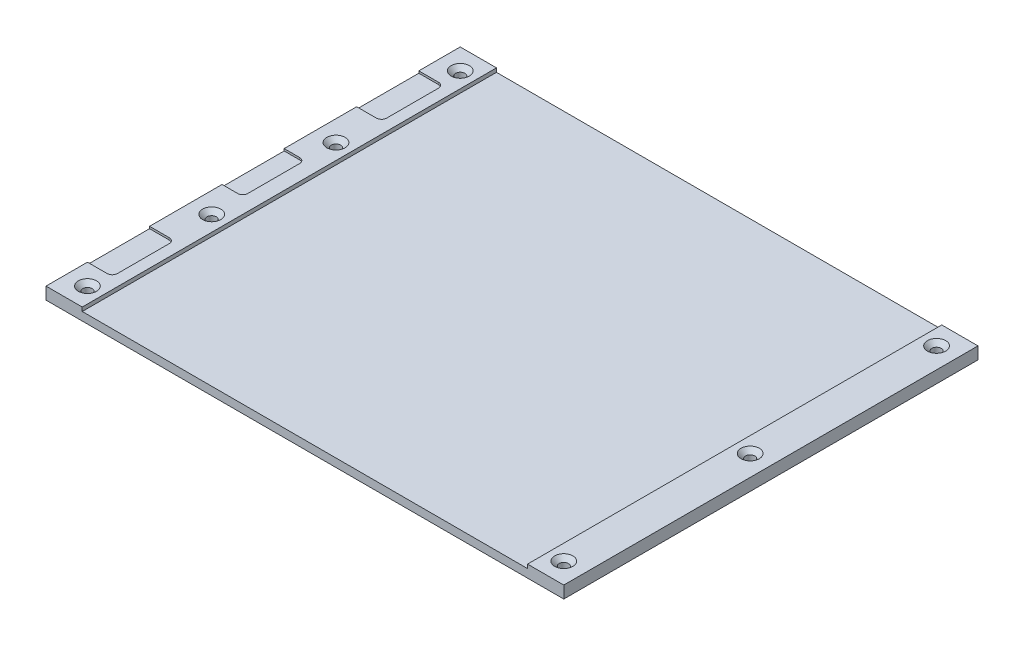
SolidWorks part; units mm, degrees
material "玻璃"
ref_plane "Front" through (0, 0, 0) normal (0, 0, 1) x (1, 0, 0)
ref_plane "Top" through (0, 0, 0) normal (0, 1, 0) x (1, 0, 0)
ref_plane "Right" through (0, 0, 0) normal (1, 0, 0) x (0, 0, -1)
sketch "Sketch1" plane through (0, 0, 0) normal (0, 0, 1) x (1, 0, 0)
  line L1 (0, 0) -> (500, 0)
  line L2 (0, 0) -> (0, 24)
  line L3 (0, 24) -> (500, 24)
  line L4 (500, 0) -> (500, 24)
  dimension "D1" = 500
  dimension "D2" = 24
extrude "Boss-Extrude1" add sketch "Sketch1" against normal blind 400
sketch "Sketch2" plane through (0, 0, 0) normal (0, 0, 1) x (1, 0, 0)
  line L0 (0, 12) -> (35, 12) construction
  line L1 (35, 16) -> (465, 16)
  line L2 (35, 16) -> (35, 8)
  line L3 (35, 8) -> (465, 8)
  line L4 (465, 16) -> (465, 8)
  line L5 (0, 24) -> (0, 0) construction
  line L6 (250, 24) -> (250, 16) construction
  line L7 (500, 24) -> (0, 24) construction
  dimension "D1" = 430
  dimension "D2" = 8
extrude "Cut-Extrude1" cut sketch "Sketch2" against normal through all
sketch "Sketch3" plane through (0, 0, 0) normal (0, 0, 1) x (1, 0, 0)
  line L0 (250, 16) -> (250, 8) construction
  line L1 (465, 16) -> (35, 16) construction
  line L2 (35, 8) -> (465, 8) construction
  line L4 (-22.4785, 12.25) -> (522.4785, 12.25)
  line L5 (-22.4785, 12.25) -> (-22.4785, 11.75)
  line L6 (-22.4785, 11.75) -> (522.4785, 11.75)
  line L7 (522.4785, 12.25) -> (522.4785, 11.75)
  line L8 (-22.4785, 12.25) -> (522.4785, 11.75) construction
  line L9 (-22.4785, 11.75) -> (522.4785, 12.25) construction
  point P6 (250, 12)
  dimension "D1" = 0.5
extrude "Cut-Extrude2" cut sketch "Sketch3" against normal through all
sketch "Sketch4" plane through (0, 0, 0) normal (-1, 0, 0) x (0, 0, 1)
  line L0 (-400, 24) -> (0, 24) construction
  line L1 (-370, 24) -> (-320, 24)
  line L2 (-370, 24) -> (-370, 0)
  line L3 (-370, 0) -> (-320, 0)
  line L4 (-320, 24) -> (-320, 0)
  line L5 (-400, 0) -> (0, 0) construction
  line L6 (-400, 24) -> (-400, 12.25) construction
  line L7 (-200, 24) -> (-200, 0) construction
  line L8 (-80, 24) -> (-80, 0)
  line L9 (-30, 0) -> (-80, 0)
  line L10 (-30, 24) -> (-30, 0)
  line L11 (-30, 24) -> (-80, 24)
  dimension "D1" = 30
  dimension "D2" = 50
sketch "Sketch12" plane through (0, 0, 0) normal (0, 0, 1) x (1, 0, 0)
  line L0 (0, 0) -> (500, 0) construction
  line L1 (-19.3284, 51.3288) -> (549.6795, 51.3288)
  line L2 (-19.3284, 51.3288) -> (-19.3284, 12)
  line L3 (-19.3284, 12) -> (549.6795, 12)
  line L4 (549.6795, 51.3288) -> (549.6795, 12)
  dimension "D1" = 12
extrude "Cut-Extrude3" cut sketch "Sketch12" against normal through all
hole_wizard "Hole wizard: hex socket semi-countersunk screw type 1" positions "Sketch14" profile "Sketch15" countersink size "M8" standard "GB" end condition through all
sketch "Sketch14" plane through (0, 11.75, 0) normal (0, 1, 0) x (1, 0, 0)
  line L0 (0, 0) -> (35, 0) construction
  line L1 (0, 400) -> (0, 0) construction
  line L3 (500, 0) -> (500, 400) construction
  line L4 (0, 400) -> (35, 400) construction
  point P0 (20, 20)
  point P2 (480, 20)
  point P4 (20, 380)
  point P6 (480, 380)
  dimension "D1" = 20
  dimension "D2" = 20
  dimension "D3" = 20
  dimension "D4" = 20
sketch "Sketch15" plane through (20, 11.75, -20) normal (1, 0, 0) x (0, 0, 1)
  line L0 (0, 0) -> (0, 11.75)
  line L1 (0, 11.75) -> (4.5, 11.75)
  line L2 (4.5, 11.75) -> (4.5, 4.3)
  line L3 (4.5, 4.3) -> (8.8, 0)
  line L5 (8.8, 0) -> (0, 0)
  line L6 (-4.5, 4.3) -> (-8.8, 0) construction
  line L11 (0, -6.35) -> (0, 107.95) construction
  dimension "通孔孔直径" = 9
  dimension "通孔孔深度" = 11.75
  dimension "近端锥形沉头孔直径" = 17.6
  dimension "近端锥形沉头孔角度" = 90
sketch "Sketch16" plane through (0, 11.75, 0) normal (0, 1, 0) x (1, 0, 0)
  line L0 (0, 400) -> (0, 0) construction
  line L1 (0, 360) -> (24, 360)
  line L2 (0, 360) -> (0, 300)
  line L3 (0, 300) -> (24, 300)
  line L4 (24, 360) -> (24, 300)
  line L5 (0, 200) -> (21.3837, 200) construction
  line L6 (24, 40) -> (24, 100)
  line L7 (0, 100) -> (24, 100)
  line L8 (0, 40) -> (0, 100)
  line L9 (0, 40) -> (24, 40)
  line L11 (20, 230) -> (0, 230)
  line L12 (20, 230) -> (20, 170)
  line L13 (20, 170) -> (0, 170)
  line L14 (0, 230) -> (0, 170)
  dimension "D1" = 24
  dimension "D2" = 60
  dimension "D3" = 200
  dimension "D4" = 60
  dimension "D5" = 20
extrude "Cut-Extrude4" cut sketch "Sketch16" against normal blind 2
fillet "Fillet1" radius 5 6 edges at (24, 10.75, -40) (24, 10.75, -100) (20, 10.75, -170) (20, 10.75, -230) (24, 10.75, -300) (24, 10.75, -360)
hole_wizard "Hole wizard: hex socket semi-countersunk screw type 2" positions "Sketch17" profile "Sketch18" countersink size "M8" standard "GB" end condition through all
sketch "Sketch17" plane through (0, 11.75, 0) normal (0, 1, 0) x (1, 0, 0)
  line L0 (0, 200) -> (10.6327, 200) construction
  line L1 (0, 230) -> (0, 170) construction
  line L3 (0, 170) -> (0, 100) construction
  line L4 (500, 0) -> (500, 400) construction
  line L5 (500, 200) -> (480, 200) construction
  point P0 (20, 140)
  point P2 (20, 260)
  point P4 (480, 200)
  dimension "D1" = 120
  dimension "D2" = 20
  dimension "D3" = 20
sketch "Sketch18" plane through (20, 11.75, -140) normal (1, 0, 0) x (0, 0, 1)
  line L0 (0, 0) -> (0, 11.75)
  line L1 (0, 11.75) -> (4.5, 11.75)
  line L2 (4.5, 11.75) -> (4.5, 4.3)
  line L3 (4.5, 4.3) -> (8.8, 0)
  line L5 (8.8, 0) -> (0, 0)
  line L6 (-4.5, 4.3) -> (-8.8, 0) construction
  line L11 (0, -6.35) -> (0, 107.95) construction
  dimension "通孔孔直径" = 9
  dimension "通孔孔深度" = 11.75
  dimension "近端锥形沉头孔直径" = 17.6
  dimension "近端锥形沉头孔角度" = 90
